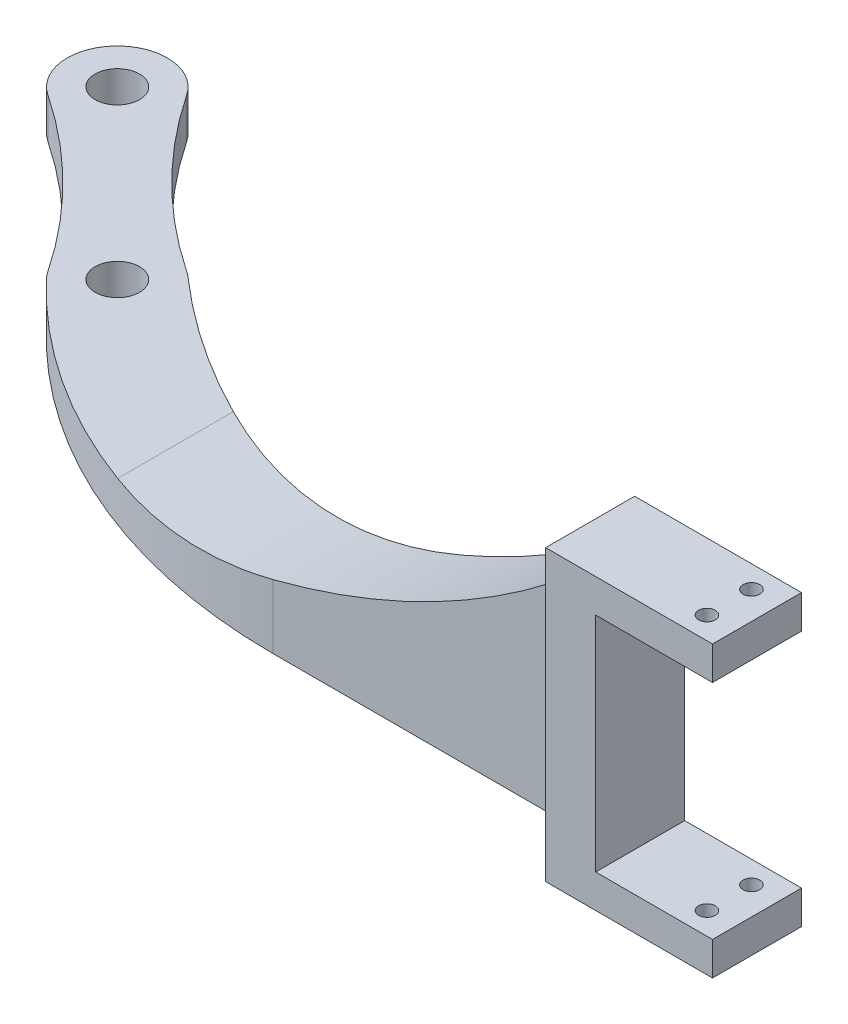
from build123d import *

# Parameters (mm, degrees)
SKETCH1_W           = 150
SKETCH1_H           = 260
BOSS_EXTRUDE1_DEPTH = 40
SKETCH2_W           = 210
SKETCH2_H           = 200
CUT_EXTRUDE1_DEPTH  = 171.073513517
SKETCH3_R           = 20
BOSS_EXTRUDE2_DEPTH = 100
SKETCH4_W           = 803.619965953
SKETCH4_H           = 20
CUT_EXTRUDE2_DEPTH  = 938.629990988
SKETCH5_R           = 7.5
CUT_EXTRUDE3_DEPTH  = 950.025816298


with BuildPart() as part:
    # Sketch1 → Boss-Extrude1 (new, symmetric)
    with BuildSketch(Plane.XY):
        Rectangle(SKETCH1_W, SKETCH1_H)
    extrude(amount=BOSS_EXTRUDE1_DEPTH, both=True)

    # Sketch2 → Cut-Extrude1 (cut, through all)
    with BuildSketch(Plane.XY.offset(40)):
        with Locations((75, 0)):
            Rectangle(SKETCH2_W, SKETCH2_H)
    extrude(amount=-CUT_EXTRUDE1_DEPTH, mode=Mode.SUBTRACT)

    # Sketch3 → Boss-Extrude2 (add, symmetric)
    with BuildSketch(Plane(origin=(0, 0, 0), x_dir=(1, 0, 0), z_dir=(0, 1, 0))):
        with BuildLine():
            Line((-75, 35), (-75, -35))
            Line((-75, -35), (-325, -35))
            ThreePointArc((-325, -35), (-519.738798114, 5.159932949), (-682.701137952, 119.086644041))
            ThreePointArc((-682.701137952, 119.086644041), (-685.176285552, 121.935272409), (-687.404051985, 124.981269115))
            ThreePointArc((-687.404051985, 124.981269115), (-749.451239008, 200.548760992), (-825.018730885, 262.595948015))
            ThreePointArc((-825.018730885, 262.595948015), (-831.819805153, 331.819805153), (-762.595948015, 325.018730885))
            ThreePointArc((-762.595948015, 325.018730885), (-700.548760992, 249.451239008), (-624.981269115, 187.404051985))
            ThreePointArc((-624.981269115, 187.404051985), (-622.594074072, 185.691949008), (-620.323675597, 183.827736695))
            ThreePointArc((-620.323675597, 183.827736695), (-436.205174947, 73.439379047), (-225, 35))
            Line((-225, 35), (-75, 35))
        make_face()
        with Locations(Location((-800, 300, 0), (0, 0, 270))):
            Circle(SKETCH3_R, mode=Mode.SUBTRACT)
        with Locations(Location((-650, 150, 0), (0, 0, 270))):
            Circle(SKETCH3_R, mode=Mode.SUBTRACT)
    extrude(amount=BOSS_EXTRUDE2_DEPTH, both=True)

    # Sketch4 → Cut-Extrude2 (cut, through all)
    with BuildSketch(Plane.XY.offset(40)):
        with BuildLine():
            Line((-845, -43.779068644), (-495, -43.779068644))
            ThreePointArc((-495, -43.779068644), (-273.03580211, -6.838732152), (-75, 100))
            Line((-75, 100), (-75, 271.543377567))
            Line((-75, 271.543377567), (-940.801447503, 271.543377567))
            Line((-940.801447503, 271.543377567), (-972.091183845, -20.942543752))
            Line((-972.091183845, -20.942543752), (-845, -43.779068644))
        make_face()
        with Locations((-476.809982977, -90)):
            Rectangle(SKETCH4_W, SKETCH4_H)
    extrude(amount=-CUT_EXTRUDE2_DEPTH, mode=Mode.SUBTRACT)

    # Sketch5 → Cut-Extrude3 (cut, through all)
    with BuildSketch(Plane(origin=(0, 130, 0), x_dir=(1, 0, 0), z_dir=(0, 1, 0))):
        with Locations(Location((50, 20, 0), (0, 0, 270))):
            Circle(SKETCH5_R)
        with Locations(Location((50, -20, 0), (0, 0, 270))):
            Circle(SKETCH5_R)
    extrude(amount=-CUT_EXTRUDE3_DEPTH, mode=Mode.SUBTRACT)


solid = part.part
